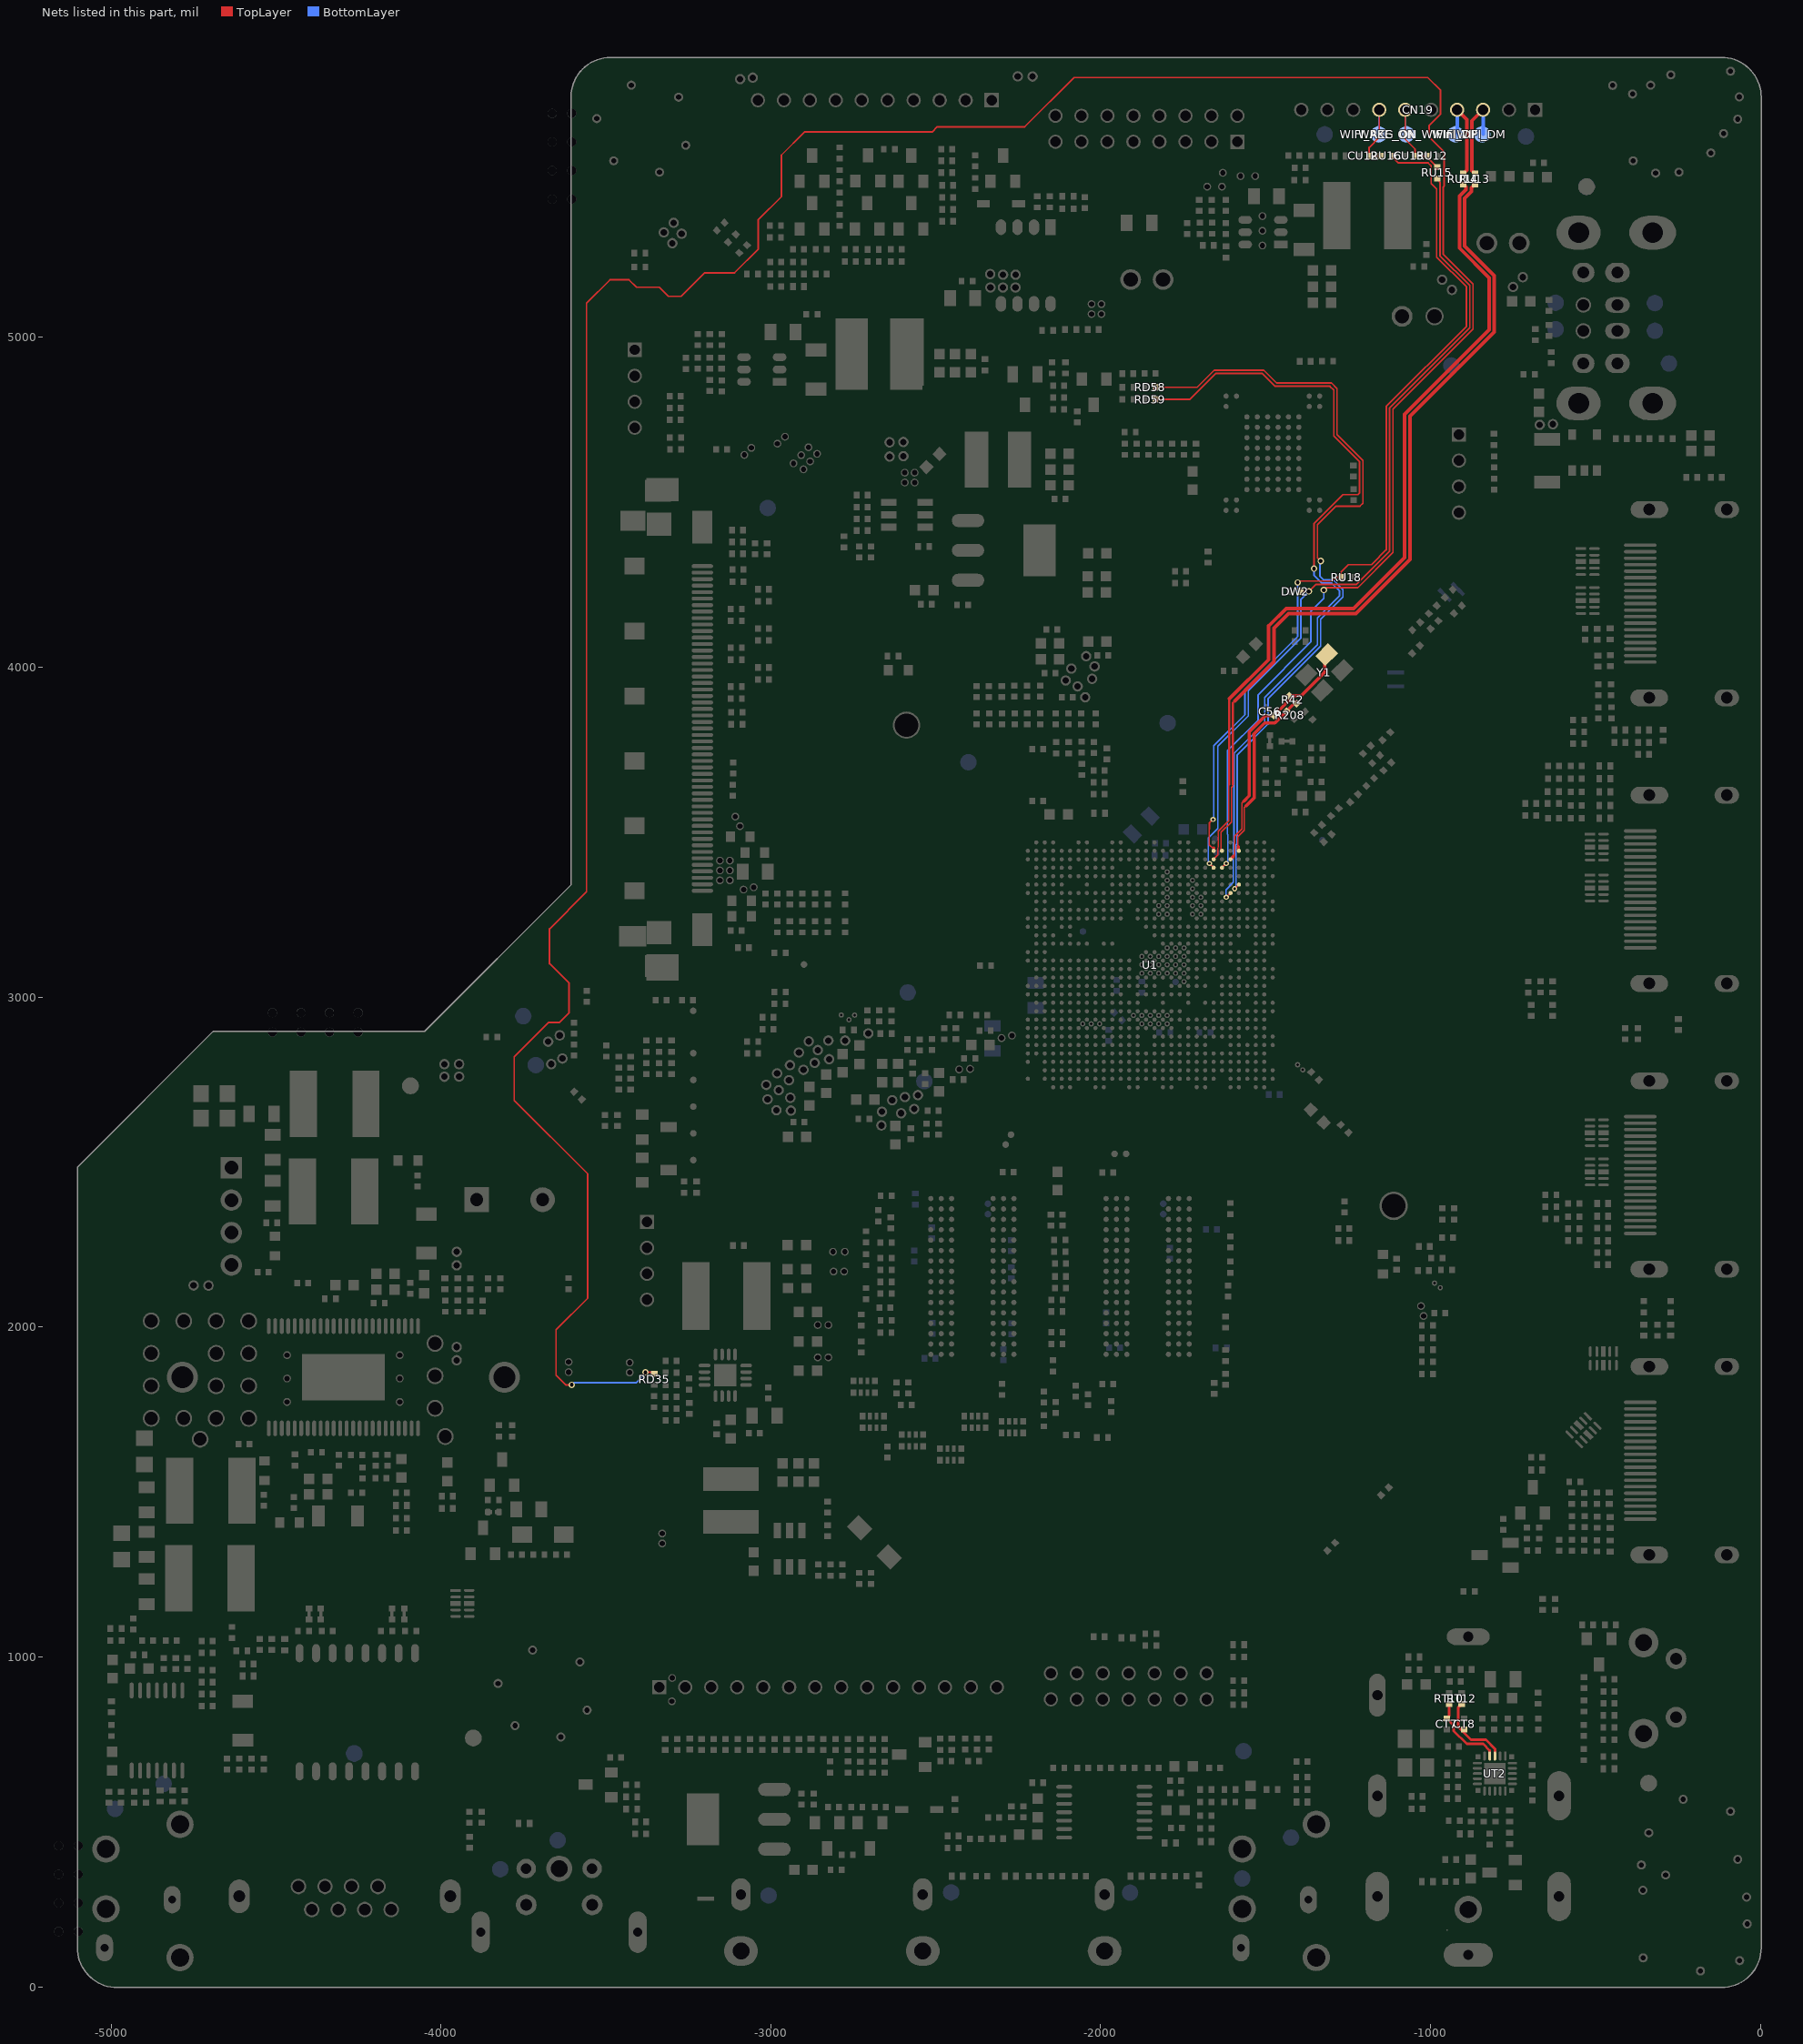
[diagram p0: the nets of this part, all layers, seen from the top]
# Altium PCB MISC86290.PcbDoc (part 29 of 31)
Units mil, origin at the board's own origin, x right, y up, seen from the top; angles counter-clockwise.
Board outline 5104.71 x 5851.49 mil, 2 copper layers (TopLayer, BottomLayer), stack 61.855 mil thick; 1026 components, 667 nets, 4280 pads, 2294 vias.

## Via types
v1: diameter 19.68, hole 11.81, TopLayer to BottomLayer, tented both sides, 1189 vias
v2: diameter 19.68/19.68 (per signal layer), hole 11.81, TopLayer to BottomLayer, tented both sides, 366 vias
v3: diameter 15.75, hole 7.87, TopLayer to BottomLayer, tented both sides, 348 vias
v4: diameter 23.62, hole 15.75, TopLayer to BottomLayer, tented both sides, 309 vias
v5: diameter 15.75/15.75 (per signal layer), hole 7.87, TopLayer to BottomLayer, tented both sides, 59 vias
v6: diameter 24/24 (per signal layer), hole 16, TopLayer to BottomLayer, tented both sides, 23 vias

## Nets (pads, with @x,y where several pads share a name; then routed paths per layer and width w, separated by ;. In a path a pad name is that pad's centre, name@x,y a point inside that pad or via, vN(x,y) a via of type N, cw(c..) or ccw(c..) an arc to the next point about the centre after c; other vN are vias at no path point) (continued)
VID1: RD35.1 U1.AG7 | length 9705.7
  TopLayer w3.94: U1.AG7@-1632.2,3392.32 v3(-1619.41,3405.12)
  TopLayer w5: v1(-3603.34,1824.66) -3621.69,1824.66 -3651,1853.97 -3651,1991.28 -3555.25,2087.03 -3555.25,2464.27 -3778,2687.02 -3778,2819.21 -3674.21,2923 -3641.52,2923 -3611.5,2953.02 -3611.5,3042 -3671,3101.5 -3671,3206.9 -3558.61,3319.29 -3558.61,5103.78 -3487.39,5175 -3430.05,5175 -3407.39,5152.34 -3337.92,5152.34 -3310.07,5124.5 -3272.21,5124.5 -3200.71,5196 -3110,5196 -3038.09,5267.91 -3038.09,5357.05 -2968,5427.14 -2968,5552.65 -2897.8,5622.85 -2510.8,5622.85 -2495.14,5638.5 -2230.14,5638.5 -2080.64,5788 -1008.61,5788 -969.54,5748.93 -969.54,5677.66 -1004,5643.2 -1004,5607 -958.61,5561.61 -958.61,5459.03 -961.53,5456.11 -961.53,5251.94 -871.09,5161.5 -871.09,5025.38 -1114.25,4782.22 -1114.25,4347.93 -1220.73,4241.45 -1316.55,4241.45 ; v1@-3380.16,1858.98 v1@-3378.91,1857.73 ; v1(-3380.16,1862.48) -3359.25,1862.48 RD35.1@-3354.5,1857.73 ; RD35.1@-3354.5,1858 RD35.1@-3354.5,1857.73 ; RD35.1@-3353.5,1857.73 RD35.1@-3354.5,1857.73
  BottomLayer w3.94: v3(-1619.41,3405.12) -1614.07,3410.46 -1614.07,3493.62
  BottomLayer w5: v1@-3596.48,1831.52 -3407.62,1831.52 v1@-3380.16,1858.98 ; -1615.95,3493.62 -1615.95,3746.98 -1522.74,3840.19 -1522.74,3916.75 -1363.04,4076.45 -1363.04,4169.46 -1323.66,4208.84 v1(-1323.66,4234.11)
VID2: RD58.1 U1.AE5 | length 2446.3
  TopLayer w3.94: v3(-1593.82,3328.35) U1.AE5@-1581.02,3341.14
  TopLayer w5: RD58.1@-1833.25,4848.95 -1707.58,4848.95 -1656.03,4900.49 -1505.54,4900.49 -1467.04,4862 -1300.5,4862 -1283.5,4845 -1283.5,4705.5 -1205,4627 -1205,4497.5 -1214,4488.5 -1286.36,4488.5 -1343,4431.86 -1343,4332 v1(-1333,4322)
  BottomLayer w3.94: v3@-1589.88,3328.35 -1589.88,3461.93 -1587.64,3464.17
  BottomLayer w5: -1587.64,3464.17 -1585.95,3465.87 -1585.95,3734.55 -1492.74,3827.76 -1492.74,3904.32 -1333.04,4064.02 -1333.04,4145.29 -1265.66,4212.67 -1265.66,4235.33 -1295.33,4265 -1325,4265 -1335,4275 -1335,4320 v1(-1333,4322)
VID3: RD59.1 U1.AD6 | length 2454.9
  TopLayer w5: RD59.1@-1833.52,4811.95 -1730.43,4811.95 -1651.89,4890.49 -1509.68,4890.49 -1471.19,4852 -1305.14,4852 -1293.5,4840.36 -1293.5,4701.36 -1215,4622.86 -1215,4528.68 -1220.18,4523.5 -1265.5,4523.5 -1353,4436 v1(-1353,4299) ; v3(-1619.41,3302.76) U1.AD6@-1606.61,3315.55
  BottomLayer w3.94: v3@-1620.2,3303.55 -1620.2,3325.58 -1597.76,3348.03 -1597.76,3468.25 ; -1596.19,3469.82 -1595.95,3470.06
  BottomLayer w5: -1596.16,3469.8 -1595.95,3470.01 ; -1595.95,3470.06 -1595.95,3738.69 -1502.74,3831.91 -1502.74,3908.47 -1343.04,4068.16 -1343.04,4149.43 -1275.66,4216.82 -1275.66,4231.18 -1299.47,4255 -1329.5,4255 -1353,4278.5 v1(-1353,4299)
VIFM: CT8.2 RT12.1 UT2.10 | length 234.1
  TopLayer w7.8: UT2.10@-804.89,699.52 -804.89,721.58
  TopLayer w8: RT12.1@-905.82,856.61 -916.66,845.76 -916.66,788.53 -877.15,749.02 -832.33,749.02 -804.89,721.58
VIFP: CT7.2 RT10.1 UT2.11 | length 243.4
  TopLayer w7.8: -840.54,736.02 -820.64,716.11 UT2.11@-820.64,699.52
  TopLayer w8: RT10.1@-943.82,856.87 -943.82,820.34 CT7.2@-950.82,813.34 -929.66,792.18 -929.66,775.32 -890.35,736.02 -840.54,736.02
WAKE_ON_WIFIN: CN19.6 CU13.1 RU12.1 RU15.1 WAKE_ON_WIFIn.1 | length 308.7
  TopLayer w5: CN19.6@-1076.93,5690.24 -1076.93,5600.93 -1047.15,5571.15 CU13.1@-1047.15,5550.24 -1014.17,5550.24 -980,5516.07 RU15.1@-980,5515.73
  BottomLayer w5: WAKE_ON_WIFIn.1@-1076.93,5615.53 CN19.6@-1076.93,5690.24
WIFI_DM: CN19.3 RU13.1 WIFI_DM.1 | length 284.9
  TopLayer w11: RU13.1@-866.15,5497.24 -874.15,5505.24 -874.15,5656.8 CN19.3@-840.71,5690.24
  BottomLayer w11: WIFI_DM.1@-840.71,5615.53 CN19.3@-840.71,5690.24
WIFI_DP: CN19.4 RU14.1 WIFI_DP.1 | length 284
  TopLayer w11: CN19.4@-919.45,5690.24 -891.4,5662.18 -890.15,5660.94 -890.15,5507.24 RU14.1@-900.15,5497.24
  BottomLayer w11: WIFI_DP.1@-919.45,5615.53 CN19.4@-919.45,5690.24
WIFI_REG_ON: RU16.2 RU18.2 U1.AJ8 | length 2696.9
  TopLayer w3.94: -1670.59,3509.09 -1670.59,3462.2 -1658.99,3450.6 U1.AJ8@-1657.8,3449.41
  TopLayer w4.92: -1670.59,3509.09 -1670.59,3527.41 v3(-1659.5,3538.5) ; v1(-1403,4257) -1398.55,4261.45 -1298.53,4261.45 -1286.98,4273 RU18.2@-1271.5,4273 -1271.5,4288.48 -1248.67,4311.31 -1179.21,4311.31 -1176.29,4314.23
  TopLayer w5: -1176.26,4314.2 -1134.25,4356.21 -1134.25,4790.51 -891.09,5033.66 -891.09,5153.21 -981.53,5243.65 -981.53,5450.53 -998,5467 -998,5519.92 -1007.08,5529 -1097.09,5529 -1117.27,5549.18 RU16.2@-1117.27,5550
  TopLayer w10: U1.AJ8@-1657.8,3443.5 -1657.06,3444.24 -1657.06,3452.53
  BottomLayer w4.92: v3(-1659.5,3538.5) -1657.22,3540.78 -1657.22,3762.21 -1562.7,3856.74 -1562.7,3933.3 -1403,4093 v1(-1403,4257) v1@-1403,4261
WIFI_REG_ON/: CN19.7 CU12.1 RU16.1 WIFI_REG_ON.1 | length 272.1
  TopLayer w5: CN19.7@-1155.67,5690.24 -1155.15,5689.72 -1155.15,5607 -1186.27,5575.89 CU12.1@-1186.27,5550 RU16.1@-1150.73,5550
  BottomLayer w5: WIFI_REG_ON.1@-1155.67,5607 CN19.7@-1155.67,5690.24
WIFI_USB_DM: RU13.2 U1.AJ7 | length 2534.5
  TopLayer w3.94: U1.AJ7@-1633.43,3444.73 -1635.16,3446.46 -1635.16,3499.61 -1603.66,3531.1 -1603.66,3635.29 -1599.47,3639.48 -1599.47,3644.03
  TopLayer w6: -1599.47,3644.03 -1599.47,3892.26 -1593.44,3898.3
  TopLayer w10: U1.AJ7@-1633.03,3445.12 -1632.2,3444.29 U1.AJ7@-1632.2,3443.5
  TopLayer w11: -1593.44,3898.3 -1474.5,4017.23 -1474.5,4118.88 -1430.77,4162.61 -1226.03,4162.61 -1062.25,4326.39 -1062.25,4760.68 -806.75,5016.18 -806.75,5187.66 -896.46,5277.37 -896.46,5421.55 -876.15,5441.85 -876.15,5453.77 RU13.2@-866.15,5463.77
WIFI_USB_DP: RU14.2 U1.AH8 | length 2560.6
  TopLayer w3.94: U1.AH8@-1657.8,3417.91 -1657.3,3418.41 -1657.3,3419.39 -1645,3431.69 -1645,3452.36 -1643.03,3454.33 -1643.03,3503.54 -1612.04,3534.54 -1612.04,3643.72 -1610.47,3645.28
  TopLayer w6: -1610.47,3645.28 -1610.47,3903.89 -1609.22,3905.14
  TopLayer w11: -1609.22,3905.14 -1490.5,4023.86 -1490.5,4125.51 -1437.4,4178.61 -1232.66,4178.61 -1078.25,4333.02 -1078.25,4767.31 -822.75,5022.81 -822.75,5181.04 -912.46,5270.75 -912.46,5428.18 -892.15,5448.48 -892.15,5455.77 RU14.2@-900.15,5463.77
WIFI_WAKE_HOST: DW2.K RU15.2 U1.AG8 | length 2560.2
  TopLayer w3.94: v3(-1670.59,3405.12) U1.AG8@-1657.8,3392.32
  TopLayer w5: DW2.K@-1394.27,4230 v1(-1369,4230) -1347.55,4251.45 -1300.47,4251.45 ; -1300.47,4251.49 -1224.83,4251.49 -1124.25,4352.07 -1124.25,4786.37 -881.09,5029.52 -881.09,5157.36 -971.53,5247.8 -971.53,5470.85 RU15.2@-980,5479.32
  BottomLayer w5: v3(-1670.59,3405.12) -1674,3408.53 -1674,3482.19 -1645,3511.19 -1645,3760.35 -1552.74,3852.62 -1552.74,3929.18 -1393.04,4088.87 -1393.04,4205.96 v1(-1369,4230)
XTALI: C56.1 R42.1 U1.AH6 Y1.3 | length 776.6
  TopLayer w3.94: -1598.14,3426.39 -1593.82,3430.71 -1593.82,3487.8 -1572.17,3509.45 -1572.17,3588.09 -1565.79,3594.46
  TopLayer w9.84: -1565.79,3594.46 -1549.55,3610.7 -1549.55,3804.41 -1500.11,3853.85 C56.1@-1475.15,3853.85 -1456.31,3872.69 -1456.31,3872.87 -1426.15,3903.02 R42.1@-1426.15,3913.36 ; R42.1@-1429.3,3913.36 R42.1@-1426.15,3913.36 ; R42.1@-1427.66,3915 R42.1@-1426.15,3915 ; R42.1@-1426.15,3916.51 R42.1@-1426.15,3915 ; Y1.3@-1314.04,4031.29 -1321,4024.33 -1321,3985 -1392.64,3913.36 R42.1@-1426.15,3913.36 ; R42.1@-1426.15,3913.36 R42.1@-1426.15,3915
  TopLayer w10: U1.AH6@-1606.61,3417.91 -1598.14,3426.39
XTALO: R42.2 R208.1 U1.AJ5 | length 548
  TopLayer w3.94: -1583.98,3456 -1583.98,3485.83 -1564.29,3505.51 -1564.29,3574.64 -1558.67,3580.26
  TopLayer w9.84: -1558.67,3580.26 -1534.71,3604.22 -1534.71,3715.24 -1534.71,3772.29 -1534.71,3790 ; -1535.21,3790 -1535.21,3798.47 -1502.47,3831.21 -1471.94,3831.21 -1410.3,3892.85 R42.2@-1402.49,3892.85
  TopLayer w10: -1582.95,3456 -1582.95,3445.43 U1.AJ5@-1581.02,3443.5
pads on no net: AI_V.0 AI_V.1 AI_V.2 AV13.0 AV14.0 AVH1.0 AVH2.0 AVH2.14 AVH3.0 AVH3.14 AVH4.0 AVI1.0 AVO1.2@-3641.74,358.27 AVO1.3@-3403.55,165.36 AVO1.3@-3879.93,165.36 AVO2.0 AVO3.0 AVO3.8 AVO4.0 AVO4.8 AVU1.0 AVU1.1@-433.45,5019.67 AVU1.2@-433.45,5098.41 AVU2.0 CA37.2@-3841,1439 CN1.0 CN2.0 CN3.0 CN16.0 CN17.0 CN19.0 CNA3.0 CNA4.0 CNA5. CNK2.0 CNK3.0 CNP2.0 CNW1.32 CNW2.32 CNW3.32 CNW12.32 EA1.0 ED1.0 ED1.5 ED1.6 ED11.0 ED11.5 ED11.6 EP1.0 EP1.5 EP1.6 H1.0 H1.1@-3582.68,885.83 H1.1@-3606.63,820.03 H1.1@-3606.63,951.62 H1.1@-3667.26,785.02 H1.1@-3667.26,986.63 H1.1@-3736.22,797.18 H1.1@-3736.22,974.48 H1.1@-3781.23,850.82 H1.1@-3781.23,920.84 H2.0 H2.1@-3283.46,5629.92 H2.1@-3307.41,5564.12 H2.1@-3368.05,5529.11 H2.1@-3437.01,5541.27 H2.1@-3482.02,5594.91 H2.1@-3482.02,5664.93 H3.0 H3.1@-94.49,433.07 H3.1@-118.44,367.27 H3.1@-118.44,498.87 H3.1@-179.08,332.26 H3.1@-179.08,533.88 H3.1@-248.03,344.42 H3.1@-248.03,521.72 H3.1@-293.04,398.06 H3.1@-293.04,468.08 H4.0 H4.1@-118.44,5642.86 H4.1@-179.08,5607.85 H5.0 H5.1@-216.86,5564.12 H5.1@-277.5,5529.11 H5.1@-346.46,5541.27 H5.1@-391.46,5594.91 H5.1@-391.46,5664.93 H6.0 H6.1@-72.03,242.28 H6.1@-115.5,306.5 H6.1@-298.61,282.23 HS1.0 HSA1.0 M1.0 M2.0 M3.0 M4.0 M5.0 M6.0 MAC.0 Manufacture_Info.0 P1(用于U1上).0 RFT1.0 S/N1.0 S/N2.0 SK1.0 SKT1.1 SKT1.2 SKT1.3 SKT1.4 SKT1.5 SKT1.6 U1.AA6 U1.AA25 U1.AA26 U1.AB1 U1.AB2 U1.AB4 U1.AB5 U1.AB6 U1.AB25 U1.AC1 U1.AC2 U1.AC3 U1.AC11 U1.AD2 U1.AD3 U1.AD4 U1.AD8 U1.AD24 U1.AE3 U1.AE16 U1.AE17 U1.AE18 U1.AE19 U1.AE20 U1.AE23 U1.AF17 U1.AF18 U1.AF19 U1.AF20 U1.AF21 U1.AF22 U1.AG3 U1.AG17 U1.AG20 U1.AG21 U1.AG22 U1.AH2 U1.AH3 U1.AH14 U1.AH16 U1.AJ21 U1.AJ22 U1.AJ23 U1.AK16 U1.AK20 U1.F1 U1.F2 U1.F5 U1.G3 U1.G10 U1.H17 U1.K29 U1.V26 U1.W25 U2.J1 U2.J9 U2.L1 U2.L9 U3.J1 U3.J9 U3.L1 U3.L9 UA1.EPAD@-4232.76,1812.31 UA1.EPAD@-4232.76,1883.18 UA1.EPAD@-4358.74,1812.31 UA1.EPAD@-4358.74,1883.18 UE1.4 UE1.5 UE1.12 UE1.13 UF1.A1 UF1.A2 UF1.A9 UF1.A10 UF1.B1 UF1.B9 UF1.B10 UF1.D6 UF1.D7 UF1.D8 UF1.E3 UF1.E4 UF1.E5 UF1.E6 UF1.E7 UF1.E8 UF1.F3 UF1.F4 UF1.F5 UF1.F6 UF1.F7 UF1.F8 UF1.G3 UF1.G5 UF1.G6 UF1.G7 UF1.G8 UF1.H3 UF1.H5 UF1.H6 UF1.H7 UF1.J3 UF1.J5 UF1.L1 UF1.L2 UF1.L9 UF1.L10 UF1.M1 UF1.M2 UF1.M9 UF1.M10 UT2.1 UT2.4 UT2.12 UT2.18 UT2.24 XXXXXX.0 XXXXXXXXXXX.0
copper on no net: | length 3421.6
  TopLayer w3.94: -1478.66,2854.92 -1475.71,2854.92
  TopLayer w5: -1888.11,2906.1 v3(-1875.32,2893.31) ; 2060.78,1384.44 2060.78,1463.18 ; 1509.88,1384.44 2241.92,1384.44 2241.92,1463.18 1509.88,1463.18 1509.88,1384.44
  BottomLayer w5: 2060.78,1166.59 2060.78,1245.33 ; 1509.88,1166.59 1509.88,1245.33 2241.92,1245.33 2241.92,1166.59 1509.88,1166.59

## Polygon pours and split planes (outlines as drawn)
GND on BottomLayer "5mil" (solid, remove dead copper, pour order 21): -2067.22,3466.04 -2084.25,3449.01 -2084.25,3358.26 -2084.25,3296.75 -2114,3267 -2344,3267 -2352.43,3267 -2413.76,3205.67 -2408.1,3200.01 -2408.1,3192.01 -2408.1,2689.9 -2518,2580 -2604,2494 -2673,2494 -2684,2494 -2729,2449 -2909,2269 -2909,2042 -2909,1600 -2539,1230 -1698,1230 -1384,1544 -1384,1736 -1384,2514 -1499,2629 -1499,2907.3 -1477.3,2929 -1496.73,2948.43 -1572.17,2948.43 -1572.17,2950.39 -1605.63,2983.86 -1605.63,3214.17 -1593.82,3225.98 -1329.02,3225.98 -1306,3249 -1306,3264 -1399,3357 -1494,3357 -1643,3506 -2027.25,3506 -2067.22,3466.04
GND on BottomLayer "5mil" (solid, remove dead copper, pour order 18): -600.37,5099 -672,5099 -680,5091 -688.5,5082.5 -696.96,5082.5 -779.5,5082.5 -810,5052 -810,5001 -780,4971 -642.7,4971 -605.36,5008.34 -594,5019.7 -594,5038 -594,5092.63 -600.37,5099
GND on BottomLayer "5" (solid, remove dead copper, pour order 31): -847,3001 -807,3001 -770,2964 -769,2963 -769,2817 -769,2362 -877,2254 -948,2325 -954,2325 -954,2394 -909,2439 -906,2442 -906,2860 -906,2944 -847,3003
GND on BottomLayer "5" (solid, remove dead copper, pour order 28): -975,3908 -1011,3872 -1011,3817 -1011,3787 -858,3634 -828,3604 -828,3183 -828,3120 -764,3056 -714,3106 -714,3176 -714,3701 -838,3825 -922,3909 -962,3909
GND on BottomLayer "5" (solid, remove dead copper, pour order 26): -1031,4390 -1031,4350 -815,4134 -752,4197 -752,4216 -752,4233 -951,4432
GND on BottomLayer "12mil" (solid, remove dead copper, pour order 30): -5101,-4 -5101,2481.95 -4689.25,2893.7 -4050.3,2893.7 -3993,2951 -3602,3342 -3602,5848 -25,5848 1,5822 1,34 -34,-1 -38,-5 -5100,-5
GND on TopLayer "5mil" (solid, remove dead copper, pour order 24): -2195.2,2829.33 -2225.71,2798.82 -2253.27,2798.82 -2305.18,2798.82 -2520,2584 -2633,2471 -2757,2471 -2790,2438 -2790,2225 -2790,2112 -2831,2071 -2852,2050 -2852,1876 -2852,1571 -2759,1478 -2570,1289 -2368,1289 -1640.78,1289 -1236.53,1693.25 -1236.53,2504.53 -1579,2847 -2177.53,2847 -2195.2,2829.33
GND on TopLayer "12mil" (solid, remove dead copper, pour order 32): -5101,-4 -5101,2481.95 -4689.25,2893.7 -4050.3,2893.7 -3993,2951 -3602,3342 -3602,5848 -25,5848 1,5822 1,34 -34,-1 -38,-5 -5100,-5
GND on TopLayer "5" (solid, remove dead copper, pour order 23): -863.09,2213.63 -625,1975.54 -625,1671 -469.75,1515.75 -430.59,1515.75 -427,1519.34 -427,1730 -369,1788 -402.76,1821.76 -402.76,2054.7 -677,2328.95 -677,2415 -434.33,2415 -431.66,2412.34 -425,2419 -425,2647.99 -430.01,2653 -538,2653 -866,2981 -1073.99,2981 -1101.44,2953.55 -1451.13,2953.55 -1472,2932.68 -1472,2836.39 -1043,2407.39 -1043,2256 -1000.63,2213.63
GND on TopLayer "5" (solid, remove dead copper, pour order 22): -1456,2735 -1419,2698 -923,2698 -763,2858 -763,3021 -763,3046 -716,3093 -714,3095 -714,3242 -451,3242 -428,3265 -428,3523 -429,3524 -749,3524 -785,3488 -1009,3264 -1009,3199 -1011,3199 -1041,3169 -1173,3169 -1184,3180 -1213,3209 -1213,3248 -1020,3441 -538,3923 -538,4024 -538,4031 -428,4141 -428,4389 -432,4393 -639,4393 -734,4298 -777,4298 -823,4252 -848,4227 -848,4162 -848,4023 -929,3942 -1004,3867 -1004,3850 -1004,3788 -1065,3727 -1499,3293 -1499,3243
GND on TopLayer "5" (solid, remove dead copper, pour order 20): -1447,4205 -1638,4014 -1638,3928 -1638,3864 -1604,3830 -1555,3781 -1511,3781 -1511,3946 -1455,4002 -1441,4016 -1441,4140
GND on TopLayer "5" (solid, remove dead copper, pour order 19): -856,5093 -870,5079 -870,4998 -787,4915 -631,4915 -584,4962 -584,4967 -584,5072 -601,5089 -612,5100 -784,5100
GND on TopLayer "5" (solid, remove dead copper, pour order 17): -789,5745 -914,5745 -943,5716 -951,5708 -951,5461 -951,5258 -941,5248 -857,5248 -830,5275 -752,5353 -752,5487 -752,5700 -762,5710
GND on TopLayer "5" (solid, remove dead copper, pour order 25): -3227,4309 -3155.69,4309 -3143.69,4321 -3135.69,4329 -3106,4329 -2933,4329 -2866,4262 -2605,4001 -2605,3934 -2605,3914 -2605,3761.01 -2436.99,3593 -2340,3593 -2312,3593 -2221,3502 -2221,3418.13 -2220.79,3417.91 -2248.32,3390.38 -2248.32,3174.8 -2578.8,3174.8 -2635,3231 -3044.75,3640.75 -3044.75,3646.38 -3044.75,3775.5 -3063.25,3794 -3133.59,3794 -3173,3833.41 -3256.41,3833.41 -3269,3846 -3269,4290 -3252,4307 -3247,4312 -3228,4312
GND on TopLayer "5" (solid, remove dead copper, pour order 27): -4433.23,1042 -4433.23,1129.77 -4357,1206 -4340,1223 -4239,1223 -4229,1233 -3573,1233 -3545,1233 -3517,1205 -3486,1174 -3224,1174 -2700,1174 -2622.89,1251.11 -2582.3,1210.52 -2582.3,1153.11 -2686.41,1049 -2695,1049 -3532,1049 -3581,1098 -3598,1115 -3679,1115 -3842,1115 -3863,1094 -4040,1094 -4055,1079 -4055,1029 -4059,1025 -4416.23,1025 -4433.23,1042
GND on TopLayer "5" (solid, remove dead copper, pour order 29): -1457.99,2737.78 -1171,2450.79 -1171,2423 -1171,2175.96 -1139.22,2144.19 -1139.22,1652.44 -1140.72,1650.94 -1197.76,1650.94 -1239.22,1692.41 -1239.22,2435.22 -1300,2496 -1511,2707 -1511,2708 -1481.22,2737.78 -1457.99,2737.78

## Keep-outs
KeepOutLayer:
  rectangle: 1509.88,787.16 1640.08,865.9
  pour cut-out: -4579,306 -4744,471 -4744,768.5 -4663.5,849 -4565,849 -4562.51,851.49 -4562.51,980 -4043,980 -3934,871 -3934,641 -3978,597 -3978,336 -4003,311 -4003,9 -4012,0 -4013,1 -4579,1
  lines w5: -5278.09,0 -8644.23,0 cw(c-8644.23,118.11) -8762.34,118.11 -8762.34,5728.35 cw(c-8644.23,5728.35) -8644.23,5846.46 -3782.02,5846.46 ; -5276.84,0 ccw(c-5276.84,118.11) -5158.73,118.11 ; -5158.73,476.38 ccw(c-5129.2,505.91) -5099.68,476.38 ; -5099.67,118.11 -5099.67,2483.36 -4689.33,2893.7 ; -4981.57,0 cw(c-4981.57,118.11) -5099.68,118.11 ccw(c-5129.2,88.58) -5158.73,118.11 ; -4980.32,0 -118.11,0 ccw(c-118.11,118.11) 0,118.11 0,5728.35 ccw(c-118.11,5728.35) -118.11,5846.46 -3484.25,5846.46 ; -4689.25,2893.7 -4048.55,2893.7 -3603.61,3338.64 -3603.61,5728.35 ; -4560.27,2893.7 ccw(c-4589.8,2923.23) -4560.27,2952.76 ; -4202,2893.7 cw(c-4172.47,2923.23) -4202,2952.76 ; -4073.09,2952.76 -4713.79,2952.76 -5158.73,2507.82 -5158.73,118.11 ; -4073.01,2952.76 -3662.67,3363.1 -3662.67,5728.35 ; -3780.78,5846.46 cw(c-3780.78,5728.35) -3662.67,5728.35 ; -3662.67,5370.08 cw(c-3633.14,5340.55) -3603.61,5370.08 ; -3485.5,5846.46 ccw(c-3485.5,5728.35) -3603.61,5728.35 ; 2060.78,787.16 2060.78,865.9 ; -3662.67,5728.35 ccw(c-3633.14,5757.87) -3603.61,5728.35 ; 1509.88,787.16 1509.88,865.9 2241.92,865.9 2241.92,787.16 1509.88,787.16
  text "KeepOutLayer" at 1662.68,808.12 h60
  text ".GKO" at 2084.49,805.21 h60

## Other copper
TopLayer:
  drawing of 222 lines, arcs and shapes, not listed
  text "TopLayer" at 1675.93,1406.78 h60
  text ".GTL" at 2085.42,1402.49 h60